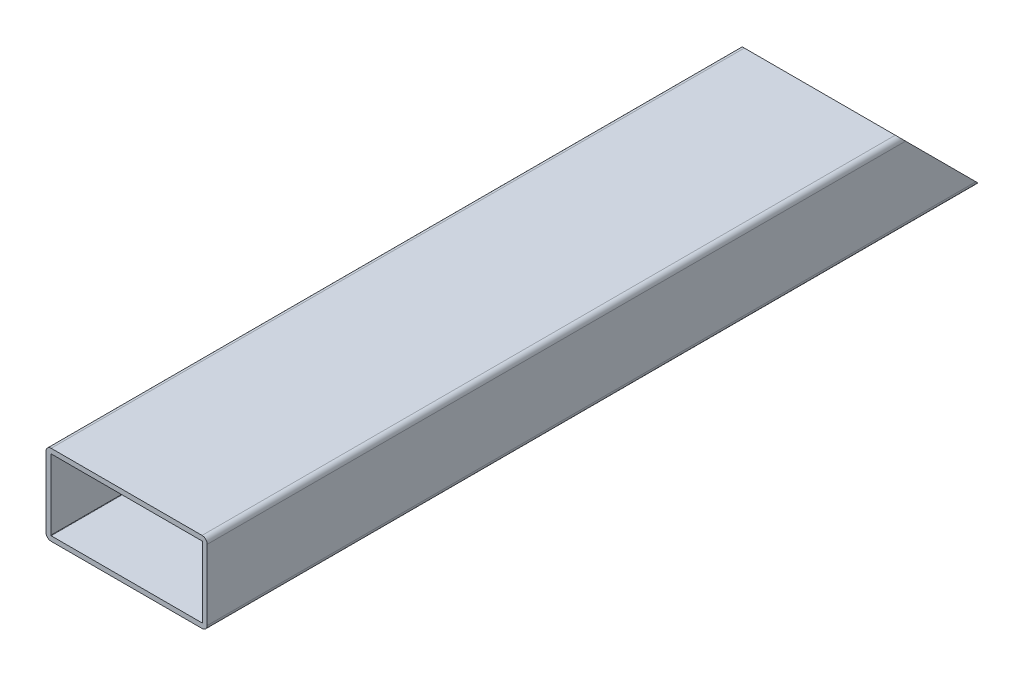
SolidWorks part; units mm, degrees
material "1023 碳钢板 (SS)"
ref_plane "前视基准面" through (0, 0, 0) normal (0, 0, 1) x (1, 0, 0)
ref_plane "上视基准面" through (0, 0, 0) normal (0, 1, 0) x (1, 0, 0)
ref_plane "右视基准面" through (0, 0, 0) normal (1, 0, 0) x (0, 0, -1)
sketch "草图1" plane through (0, 0, 0) normal (0, 0, 1) x (1, 0, 0)
  line L0 (-46.8, 22) -> (46.8, 22)
  line L1 (-46.8, 25) -> (46.8, 25)
  line L2 (-50, 21.8) -> (-50, -21.8)
  line L3 (-46.8, -25) -> (46.8, -25)
  line L4 (50, 21.8) -> (50, -21.8)
  line L5 (-50, 25) -> (50, -25) construction
  line L6 (-50, -25) -> (50, 25) construction
  line L7 (47, 21.8) -> (47, -21.8)
  line L8 (-46.8, -22) -> (46.8, -22)
  line L9 (-47, 21.8) -> (-47, -21.8)
  line L10 (-50, 25) -> (50, 25) construction
  line L11 (-50, 25) -> (-50, -25) construction
  line L12 (-50, -25) -> (50, -25) construction
  line L13 (50, 25) -> (50, -25) construction
  line L14 (-47, 22) -> (47, 22) construction
  line L15 (47, 22) -> (47, -22) construction
  line L16 (-47, -22) -> (47, -22) construction
  line L17 (-47, 22) -> (-47, -22) construction
  arc A0 (-46.8, 25) -> (-50, 21.8) centre (-46.8, 21.8) ccw
  arc A1 (-50, -21.8) -> (-46.8, -25) centre (-46.8, -21.8) ccw
  arc A2 (46.8, -25) -> (50, -21.8) centre (46.8, -21.8) ccw
  arc A3 (46.8, 25) -> (50, 21.8) centre (46.8, 21.8) cw
  arc A4 (46.8, 22) -> (47, 21.8) centre (46.8, 21.8) cw
  arc A5 (47, -21.8) -> (46.8, -22) centre (46.8, -21.8) cw
  arc A6 (-46.8, -22) -> (-47, -21.8) centre (-46.8, -21.8) cw
  arc A7 (-46.8, 22) -> (-47, 21.8) centre (-46.8, 21.8) ccw
  point P0 (0, 0)
  dimension "D4" = 3.2
  dimension "D5" = 0.2
  dimension "D1" = 100
  dimension "D2" = 50
  dimension "D3" = 3
extrude "凸台-拉伸1" add sketch "草图1" along normal blind 500 contours L0 L9 L8 L7 | L2 A1 L3 A2 L4 A3 L1 A0
sketch "草图3" plane through (50, 0, 0) normal (1, 0, 0) x (0, 0, -1)
  line L0 (-70, 25) -> (-20, -25)
  line L1 (-500, 25) -> (0, 25) construction
  line L2 (-500, -25) -> (0, -25) construction
  line L3 (-70, 25) -> (18.0103, 25)
  line L4 (18.0103, 25) -> (18.0103, -26.4233)
  line L5 (18.0103, -26.4233) -> (-20, -25)
  dimension "D1" = 45
  dimension "D2" = 480
extrude "切除-拉伸1" cut sketch "草图3" against normal blind 480
